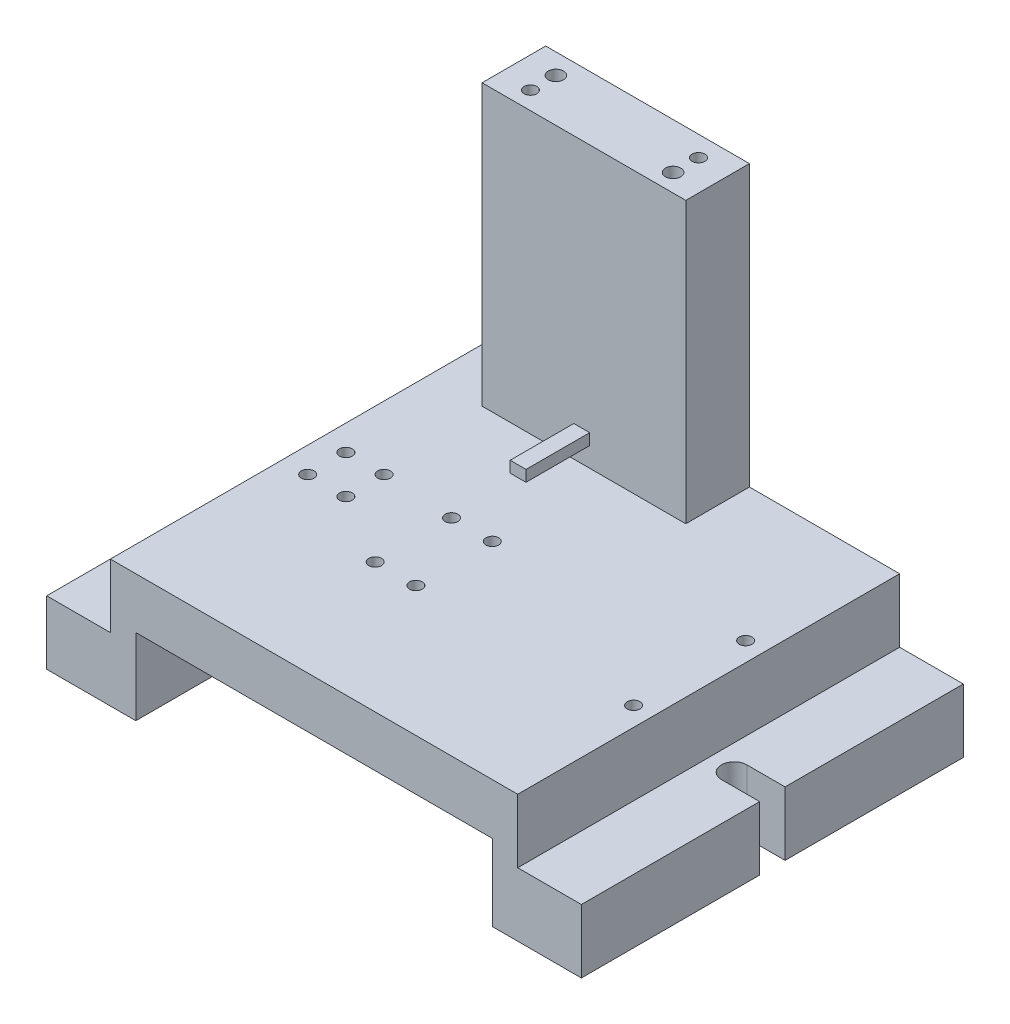
from build123d import *

# Parameters (mm, degrees)
BOSS_EXTRUDE1_DEPTH        = 150
CUT_EXTRUDE1_DEPTH         = 260.277843249
M6_TAPPED_HOLE1_D          = 5
M6_TAPPED_HOLE1_DEPTH      = 15
M6_TAPPED_HOLE1_TIP        = 1.502151548
SKETCH13_W                 = 80
SKETCH13_H                 = 25
BOSS_EXTRUDE2_DEPTH        = 110
M6_TAPPED_HOLE2_D          = 5
M6_TAPPED_HOLE2_DEPTH      = 15
M6_TAPPED_HOLE2_TIP        = 1.502151548
F_6_0MM_DOWEL_HOLE_1_D     = 6
F_6_0MM_DOWEL_HOLE_1_DEPTH = 15
F_6_0MM_DOWEL_HOLE_1_TIP   = 1.802581857
SKETCH20_W                 = 6.227014718
SKETCH20_H                 = 4.395715082
BOSS_EXTRUDE3_DEPTH        = 25


with BuildPart() as part:
    # Sketch1 → Boss-Extrude1 (new body)
    with BuildSketch(Plane.XY):
        Polygon((0, 0), (0, 25), (25, 25), (25, 50), (185, 50), (185, 25), (210, 25), (210, 0), (175, 0), (175, 30), (35, 30), (35, 0), align=None)
    extrude(amount=BOSS_EXTRUDE1_DEPTH)

    # Sketch9 → Cut-Extrude1 (cut, through all)
    with BuildSketch(Plane(origin=(0, 25, 0), x_dir=(1, 0, 0), z_dir=(0, 1, 0))):
        with BuildLine():
            Line((210, -70), (210, -80))
            Line((210, -80), (195, -80))
            ThreePointArc((195, -80), (190, -75), (195, -70))
            Line((195, -70), (210, -70))
        make_face()
        with BuildLine():
            Line((15, -70), (0, -70))
            Line((0, -70), (0, -80))
            Line((0, -80), (15, -80))
            ThreePointArc((15, -80), (20, -75), (15, -70))
        make_face()
    extrude(amount=-CUT_EXTRUDE1_DEPTH, mode=Mode.SUBTRACT)

    # M6 Tapped Hole1
    with Locations(Plane(origin=(0, 50, 0), x_dir=(1, 0, 0), z_dir=(0, 1, 0))):
        with Locations((35, -82.5), (35, -67.5), (50, -67.5), (50, -82.5), (78, -69), (78, -99), (94, -69), (94, -99), (177.5, -97), (177.5, -53)):
            Hole(M6_TAPPED_HOLE1_D / 2, depth=M6_TAPPED_HOLE1_DEPTH)
            with Locations((0, 0, -(M6_TAPPED_HOLE1_DEPTH + M6_TAPPED_HOLE1_TIP / 2))):  # 118° drill point
                Cone(0, M6_TAPPED_HOLE1_D / 2, M6_TAPPED_HOLE1_TIP, mode=Mode.SUBTRACT)

    # Sketch13 → Boss-Extrude2 (add)
    with BuildSketch(Plane(origin=(0, 50, 0), x_dir=(1, 0, 0), z_dir=(0, 1, 0))):
        with Locations((86, -12.5)):
            Rectangle(SKETCH13_W, SKETCH13_H)
    extrude(amount=BOSS_EXTRUDE2_DEPTH)

    # M6 Tapped Hole2
    with Locations(Plane(origin=(0, 160, 0), x_dir=(1, 0, 0), z_dir=(0, 1, 0))):
        with Locations((58, -18), (114, -8)):
            Hole(M6_TAPPED_HOLE2_D / 2, depth=M6_TAPPED_HOLE2_DEPTH)
            with Locations((0, 0, -(M6_TAPPED_HOLE2_DEPTH + M6_TAPPED_HOLE2_TIP / 2))):  # 118° drill point
                Cone(0, M6_TAPPED_HOLE2_D / 2, M6_TAPPED_HOLE2_TIP, mode=Mode.SUBTRACT)

    # Ø6.0mm dowel hole 1
    with Locations(Plane(origin=(0, 160, 0), x_dir=(1, 0, 0), z_dir=(0, 1, 0))):
        with Locations((58, -8), (114, -18)):
            Hole(F_6_0MM_DOWEL_HOLE_1_D / 2, depth=F_6_0MM_DOWEL_HOLE_1_DEPTH)
            with Locations((0, 0, -(F_6_0MM_DOWEL_HOLE_1_DEPTH + F_6_0MM_DOWEL_HOLE_1_TIP / 2))):  # 118° drill point
                Cone(0, F_6_0MM_DOWEL_HOLE_1_D / 2, F_6_0MM_DOWEL_HOLE_1_TIP, mode=Mode.SUBTRACT)

    # Sketch20 → Boss-Extrude3 (add)
    with BuildSketch(Plane.XY.offset(25)):
        with Locations((85.142135624, 59.920221849)):
            Rectangle(SKETCH20_W, SKETCH20_H)
    extrude(amount=BOSS_EXTRUDE3_DEPTH)


solid = part.part
